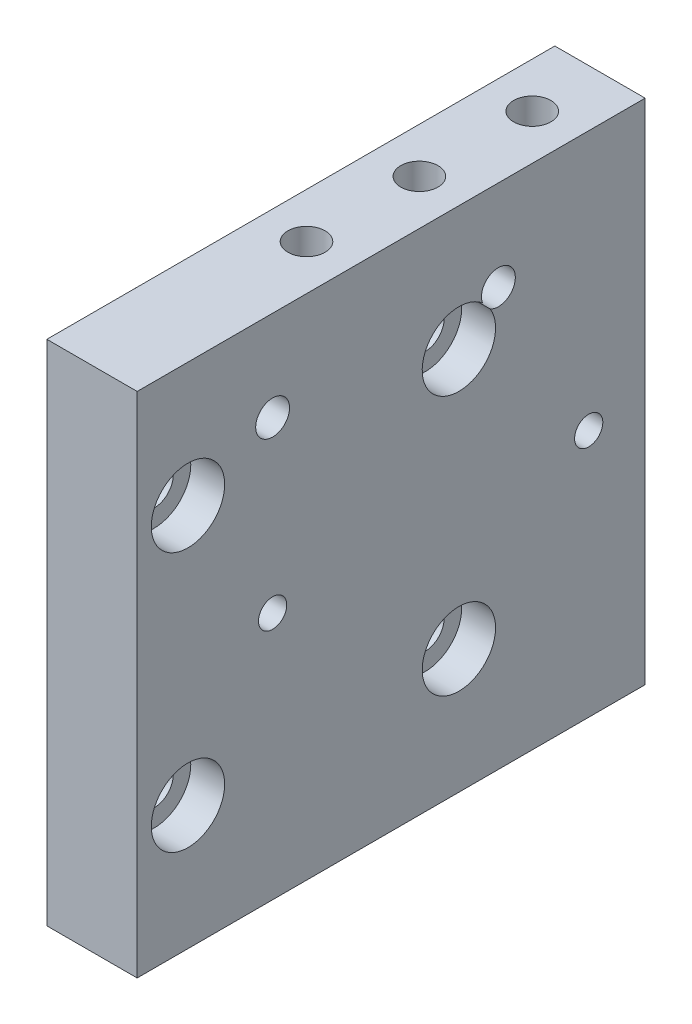
from build123d import *

# Parameters (mm, degrees)
SKETCH_1_W                                        = 45
SKETCH_1_H                                        = 45
BOSS_EXTRUDE_1_DEPTH                              = 8
M3_HEX_SOCKET_CAP_SCREW_COUNTERBORE_1_D           = 3.4
M3_HEX_SOCKET_CAP_SCREW_COUNTERBORE_1_CBORE_D     = 6.5
M3_HEX_SOCKET_CAP_SCREW_COUNTERBORE_1_CBORE_DEPTH = 3
LINEAR_PATTERN_1_COUNT                            = 2
LINEAR_PATTERN_1_PITCH                            = 23
LINEAR_PATTERN_2_COUNT                            = 2
LINEAR_PATTERN_2_PITCH                            = 24
LINEAR_PATTERN_2_COPY_1_D                         = 3.4
LINEAR_PATTERN_2_COPY_1_CBORE_D                   = 6.5
LINEAR_PATTERN_2_COPY_1_CBORE_DEPTH               = 3
LINEAR_PATTERN_5_COUNT                            = 3
LINEAR_PATTERN_5_PITCH                            = 10
M3_TAPPED_HOLE_1_D                                = 2.5
LINEAR_PATTERN_6_COUNT                            = 2
LINEAR_PATTERN_6_PITCH                            = 28
F_3_0_3_HOLE_1_D                                  = 3
LINEAR_PATTERN_8_COUNT                            = 2
LINEAR_PATTERN_8_PITCH                            = 20


with BuildPart() as part:
    # Sketch 1 → Boss-Extrude 1 (new body)
    with BuildSketch(Plane(origin=(0, 0, 0), x_dir=(0, 0, -1), z_dir=(1, 0, 0))):
        Rectangle(SKETCH_1_W, SKETCH_1_H)
    extrude(amount=BOSS_EXTRUDE_1_DEPTH)

    # M3 Hex Socket Cap Screw Counterbore 1 (through all)
    with Locations(Plane(origin=(8, 0, 0), x_dir=(0, 0, -1), z_dir=(1, 0, 0))):
        with Locations((-18, 11.5)):
            m3_hex_socket_cap_screw_counterbore_1 = CounterBoreHole(M3_HEX_SOCKET_CAP_SCREW_COUNTERBORE_1_D / 2, M3_HEX_SOCKET_CAP_SCREW_COUNTERBORE_1_CBORE_D / 2, M3_HEX_SOCKET_CAP_SCREW_COUNTERBORE_1_CBORE_DEPTH)

    # Linear Pattern 1: M3 Hex Socket Cap Screw Counterbore 1 ×2
    with Locations(*[(0, -i * LINEAR_PATTERN_1_PITCH, 0) for i in range(1, LINEAR_PATTERN_1_COUNT)]):
        add(m3_hex_socket_cap_screw_counterbore_1, mode=Mode.SUBTRACT)

    # Linear Pattern 2: M3 Hex Socket Cap Screw Counterbore 1 ×2
    with Locations(*[(0, 0, -i * LINEAR_PATTERN_2_PITCH) for i in range(1, LINEAR_PATTERN_2_COUNT)]):
        add(m3_hex_socket_cap_screw_counterbore_1, mode=Mode.SUBTRACT)

    # Linear Pattern 2 copy 1 (through all)
    with Locations(Plane(origin=(8, -23, -24), x_dir=(0, 0, -1), z_dir=(1, 0, 0))):
        with Locations((-18, 11.5)):
            CounterBoreHole(LINEAR_PATTERN_2_COPY_1_D / 2, LINEAR_PATTERN_2_COPY_1_CBORE_D / 2, LINEAR_PATTERN_2_COPY_1_CBORE_DEPTH)

    # Sketch 6 → M4 Tapped Hole 1 (revolve, cut)
    with BuildSketch(Plane(origin=(4, 22.5, -16.5), x_dir=(0, 0, 1), z_dir=(1, 0, 0))):
        Polygon((0, 0), (0, 11.091420021), (1.65, 10.1), (1.65, 0), align=None)
    m4_tapped_hole_1 = revolve(axis=Axis((4, 28.85, -16.5), (0, -1, 0)), mode=Mode.SUBTRACT)

    # Linear Pattern 5: M4 Tapped Hole 1 ×3
    with Locations(*[(0, 0, i * LINEAR_PATTERN_5_PITCH) for i in range(1, LINEAR_PATTERN_5_COUNT)]):
        add(m4_tapped_hole_1, mode=Mode.SUBTRACT)

    # M3 Tapped Hole 1 (through all)
    with Locations(Plane(origin=(8, 0, 0), x_dir=(0, 0, -1), z_dir=(1, 0, 0))):
        with Locations((17.5, -0.5)):
            m3_tapped_hole_1 = Hole(M3_TAPPED_HOLE_1_D / 2)

    # Linear Pattern 6: M3 Tapped Hole 1 ×2
    with Locations(*[(0, 0, i * LINEAR_PATTERN_6_PITCH) for i in range(1, LINEAR_PATTERN_6_COUNT)]):
        add(m3_tapped_hole_1, mode=Mode.SUBTRACT)

    # Ø3.0 (3) Hole 1 (through all)
    with Locations(Plane(origin=(8, 0, 0), x_dir=(0, 0, -1), z_dir=(1, 0, 0))):
        with Locations((-10.5, 14.5)):
            f_3_0_3_hole_1 = Hole(F_3_0_3_HOLE_1_D / 2)

    # Linear Pattern 8: Ø3.0 (3) Hole 1 ×2
    with Locations(*[(0, 0, -i * LINEAR_PATTERN_8_PITCH) for i in range(1, LINEAR_PATTERN_8_COUNT)]):
        add(f_3_0_3_hole_1, mode=Mode.SUBTRACT)


solid = part.part
